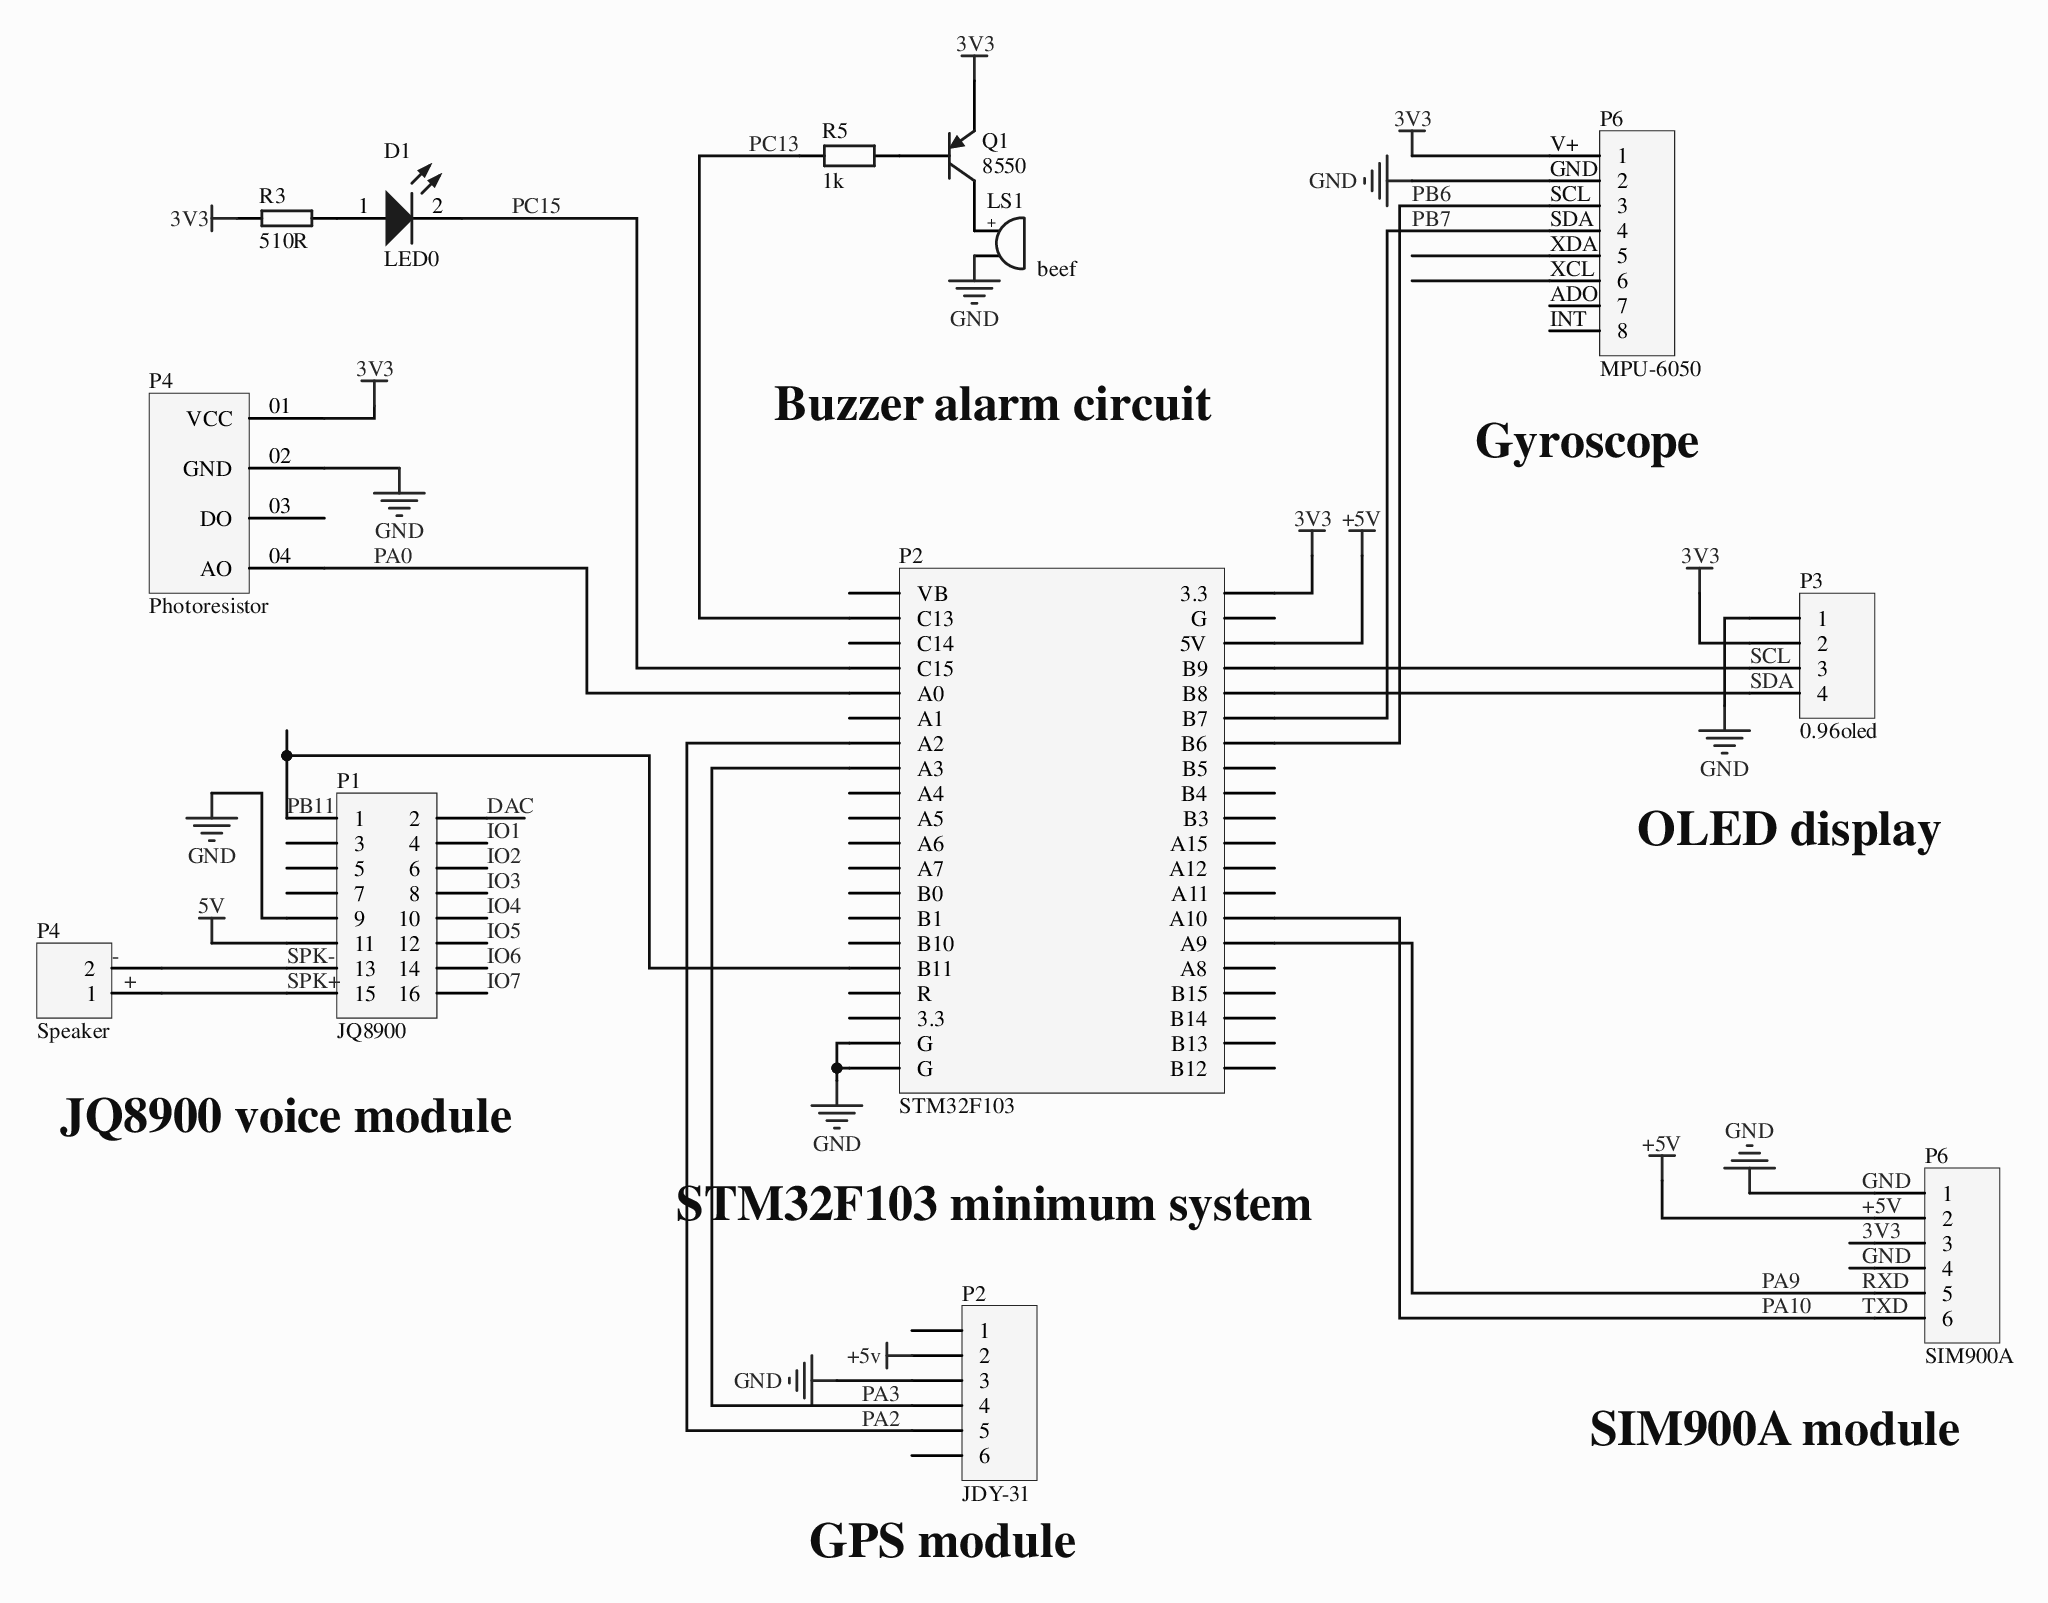
[diagram p0: MISC84382-8.SchDoc]
# Altium project MISC84382-6.PrjPcb
1 sheet, 13 parts. Net scope: global (net labels, ports and power ports of the same name join across sheets).
Board file: MISC84382.PcbDoc

## Sheet MISC84382-8.SchDoc
size A3

### Parts
(Parts that share a designator on the sheet are numbered #1, #2 ... from top to bottom, then left to right.)
D1  LED0  [my0603LED]
LS1  beef  [PIN2]
P1  JQ8900  [HDR2X8]
P2#1  STM32F103  [STM32核心板]
P2#2  JDY-31  [HDR1X6]
P3  0.96oled  [HDR1X4]
P4#1  Photoresistor  [HDR1X4]
P4#2  Speaker  [HDR1X2]
P6#1  MPU-6050  [HDR1X8]
P6#2  SIM900A  [HDR1X6]
Q1  8550  [TO-92A]
R3  510R  [my0603]
R5  1k  [my0603]

### Nets
3V3: P2#1.39(3.3) P3.2 P4#1.01(VCC) P6#1.1 P6#2.3 Q1.1(E) R3.2
5V: P1.11
+5V: P2#1.35(5V) P2#2.2 P6#2.2
GND: LS1.2 P1.9 P2#1.2(G) P2#1.4(G) P2#2.3 P3.1 P4#1.02(GND) P6#1.2 P6#2.1 P6#2.4
DAC: P1.2
IO1: P1.4
IO2: P1.6
IO3: P1.8
IO4: P1.10
IO5: P1.12
IO6: P1.14
IO7: P1.16
PA0: P2#1.32(A0) P4#1.04(AO)
PA2: P2#1.28(A2) P2#2.5
PA3: P2#1.26(A3) P2#2.4
PA9: P2#1.11(A9) P6#2.5  [also labelled RXD]
PA10: P2#1.13(A10) P6#2.6  [also labelled TXD]
PB6: P2#1.27(B6) P6#1.3
PB7: P2#1.29(B7) P6#1.4
PB11: P1.1 P2#1.10(B11)
PC13: P2#1.38(C13) R5.1
PC15: D1.2(K) P2#1.34(C15)
SCL: P2#1.33(B9) P3.3
SDA: P2#1.31(B8) P3.4
SPK+: P1.15 P4#2.1
SPK-: P1.13 P4#2.2
NetD1_1: D1.1(A) R3.1
NetLS1_1: LS1.1 Q1.3(C)
NetQ1_2: Q1.2(B) R5.2

Not connected (* = marked no-connect by the designer): P1 3 5 7; P2#1 3(B13) 5(B14) 6(3.3) 7(B15) 8(R) 9(A8) 12(B10) 14(B1) 15(A11) 16(B0) 17(A12) 18(A7) 19(A15) 20(A6) 21(B3) 22(A5) 23(B4) 24(A4) 25(B5) 30(A1) 36(C14) 37(G) 40(VB) B12; P2#2 1 6; P4#1 03(DO); P6#1 5 6 7 8

### Notes on the sheet
- (near P6#1) V+
- (near P6#1) GND
- (near P6#1) SCL
- (near P6#1) SDA
- (near P6#1) XDA
- (near P6#1) XCL
- (near P6#1) ADO
- (near P6#1) INT
- Buzzer alarm circuit
- (near P6#1) Gyroscope
- OLED display
- JQ8900 voice module
- STM32F103 minimum system
- (near P6#2) SIM900A module
- (near P2#2) GPS module
- Labels drawn without touching a wire or pin: +, -

### Library data of the parts
D1 = LED0: Typical INFRARED GaAs LED
LS1 = BEEP: Buzzer; BOM名称: Buzzer
P1 = Header 8X2: Header, 8-Pin, Dual row; LatestRevisionDate: 17-Jul-2002; LatestRevisionNote: Re-released for DXP Platform.; Publisher: Altium Limited
P2#1 = Header 20X2: Header, 20-Pin, Dual row; LatestRevisionDate: 17-Jul-2002; LatestRevisionNote: Re-released for DXP Platform.; Publisher: Altium Limited
P2#2 P6#2 = Header 6: Header, 6-Pin; LatestRevisionDate: 17-Jul-2002; LatestRevisionNote: Re-released for DXP Platform.; Publisher: Altium Limited
P3 = Header 4: Header, 4-Pin; LatestRevisionDate: 17-Jul-2002; LatestRevisionNote: Re-released for DXP Platform.; Publisher: Altium Limited
P4#1 = Component_1
P4#2 = Header 2: Header, 2-Pin; LatestRevisionDate: 17-Jul-2002; LatestRevisionNote: Re-released for DXP Platform.; Publisher: Altium Limited
P6#1 = Header 8: Header, 8-Pin; LatestRevisionDate: 17-Jul-2002; LatestRevisionNote: Re-released for DXP Platform.; Publisher: Altium Limited
Q1 = 2N3906: PNP General Purpose Amplifier; Published: 8-Jun-2000; LatestRevisionDate: 15-Jan-2003; LatestRevisionNote: PCB Footprint 'BCY-W3/D4.7' replaced; DatasheetVersion: 1997; PackageVersion: Sep-1998; PackageReference: TO-92A; PackageDescription: TO, Flat Index; 3 In-Line, Axial Leads; Body Dia. 4.5mm; Leads 0.51 x 0.48 mm (max); ComponentLink1Description: Manufacturer Link; ComponentLink2Description: Datasheet; ComponentLink2URL: http://www.fairchildsemi.com/ds/2N%2F2N3906.pdf; Publisher: Altium Limited
R3 = R
R5 = R: SMD resistor; BOM名称: SMD resistor